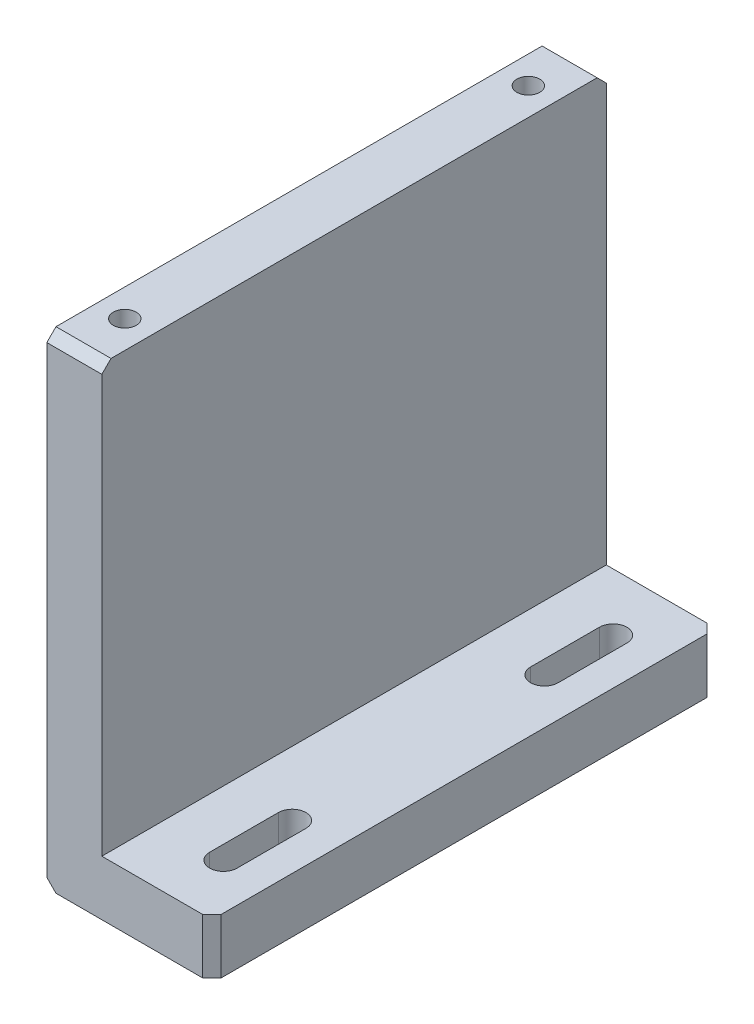
SolidWorks part; units mm, degrees
material "Q235-A"
ref_plane "Front Plane" through (0, 0, 0) normal (0, 0, 1) x (1, 0, 0)
ref_plane "Top Plane" through (0, 0, 0) normal (0, 1, 0) x (1, 0, 0)
ref_plane "Right Plane" through (0, 0, 0) normal (1, 0, 0) x (0, 0, -1)
sketch "Sketch1" plane through (0, 0, 0) normal (0, 0, 1) x (1, 0, 0)
  line L0 (-38.6012, 51.7778) -> (-38.6012, -53.2222)
  line L1 (-38.6012, -53.2222) -> (-2.6012, -53.2222)
  line L2 (-2.6012, -53.2222) -> (-2.6012, -41.2222)
  line L3 (-2.6012, -41.2222) -> (-26.6012, -41.2222)
  line L4 (-26.6012, -41.2222) -> (-26.6012, 51.7778)
  line L5 (-26.6012, 51.7778) -> (-38.6012, 51.7778)
  dimension "D1" = 36
  dimension "D2" = 105
  dimension "D3" = 12
  dimension "D4" = 12
extrude "Boss-Extrude1" add sketch "Sketch1" along normal blind 110
chamfer "Chamfer1" distance 2 angle 45 5 edges at (-38.6012, -53.2222, 55) (-2.6012, -47.2222, 0) (-2.6012, -47.2222, 110) (-32.6012, 51.7778, 0) (-32.6012, 51.7778, 110)
sketch "Sketch2" plane through (0, -41.2222, 0) normal (0, 1, 0) x (1, 0, 0)
  line L0 (7.2617, -55) -> (-54.2127, -55) construction
  line L1 (-12.6012, -97.5) -> (-12.6012, -82.5) construction
  line L2 (-15.6012, -97.5) -> (-15.6012, -82.5)
  line L3 (-9.6012, -97.5) -> (-9.6012, -82.5)
  line L4 (-38.6012, -108) -> (-38.6012, -2) construction
  line L5 (-4.6012, -110) -> (-26.6012, -110) construction
  line L6 (-12.6012, -12.5) -> (-12.6012, -27.5) construction
  line L7 (-15.6012, -12.5) -> (-15.6012, -27.5)
  line L8 (-9.6012, -12.5) -> (-9.6012, -27.5)
  arc A0 (-15.6012, -97.5) -> (-9.6012, -97.5) centre (-12.6012, -97.5) ccw
  arc A1 (-9.6012, -82.5) -> (-15.6012, -82.5) centre (-12.6012, -82.5) ccw
  arc A2 (-15.6012, -12.5) -> (-9.6012, -12.5) centre (-12.6012, -12.5) cw
  arc A3 (-9.6012, -27.5) -> (-15.6012, -27.5) centre (-12.6012, -27.5) cw
  point P4 (-12.6012, -90)
  point P15 (-12.6012, -20)
  dimension "D2" = 3
  dimension "D4" = 12.5
  dimension "D1" = 15
  dimension "D3" = 26
extrude "Cut-Extrude1" cut sketch "Sketch2" against normal through all
sketch "Sketch3" plane through (0, 51.7778, 0) normal (0, 1, 0) x (1, 0, 0)
  line L0 (-32.6012, -99) -> (-32.6012, -11)
  line L1 (-26.6012, -110) -> (-38.6012, -110) construction
  dimension "D1" = 88
  dimension "D2" = 11
hole_wizard "M6 Tapped Hole1" positions "Sketch4" profile "Sketch5" tap size "M6" standard "GB"
sketch "Sketch4" plane through (0, 51.7778, 0) normal (0, 1, 0) x (1, 0, 0)
  point P0 (-32.6012, -99)
  point P3 (-32.6012, -11)
sketch "Sketch5" plane through (-32.6012, 51.7778, 99) normal (1, 0, 0) x (0, 0, 1)
  line L0 (0, 0) -> (0, 12)
  line L1 (0, 12) -> (2.5, 10.4978)
  line L2 (2.5, 10.4978) -> (2.5, 0)
  line L5 (2.5, 0) -> (0, 0)
  line L10 (0, 12) -> (-2.5, 10.4978) construction
  line L11 (0, -6.35) -> (0, 107.95) construction
  dimension "螺纹孔钻头直径" = 5
  dimension "螺纹孔钻头深度" = 12
  dimension "导头角度" = 118
cosmetic thread "Cosmetic thread 1" parameters "D1"=10.4978, "D2"=6
cosmetic thread "Cosmetic thread 2" parameters "D1"=10.4978, "D2"=6
